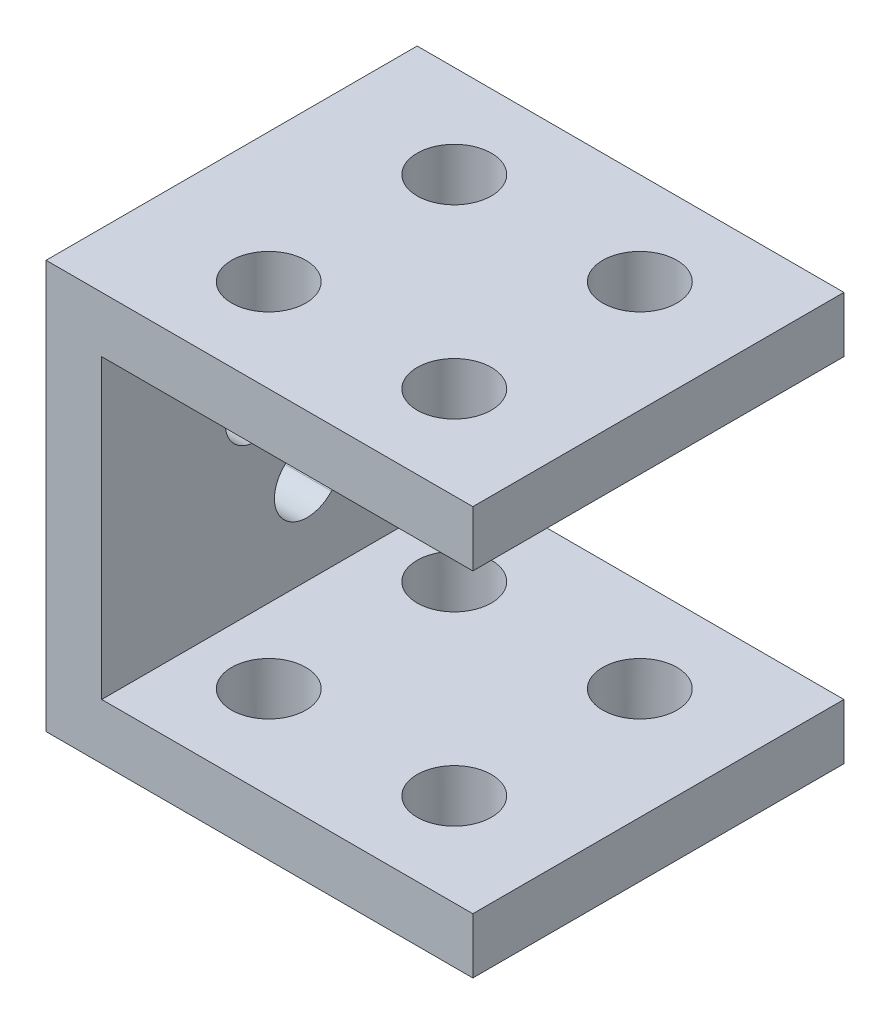
from build123d import *

# Parameters (mm, degrees)
BOSS_EXTRUDE1_DEPTH = 100
SKETCH2_R           = 10
CUT_EXTRUDE1_DEPTH  = 500
CUT_EXTRUDE2_DEPTH  = 500


with BuildPart() as part:
    # Sketch1 → Boss-Extrude1 (new body)
    with BuildSketch(Plane.XY):
        Polygon((0, 0), (100, 0), (100, -15), (-15, -15), (-15, 95), (100, 95), (100, 80), (0, 80), align=None)
    extrude(amount=BOSS_EXTRUDE1_DEPTH)

    # Sketch2 → Cut-Extrude1 (cut)
    with BuildSketch(Plane(origin=(0, 95, 0), x_dir=(1, 0, 0), z_dir=(0, 1, 0))):
        with Locations(Location((20, -25, 0), (0, 0, 270))):
            Circle(SKETCH2_R)
        with Locations(Location((70, -25, 0), (0, 0, 270))):
            Circle(SKETCH2_R)
        with Locations(Location((20, -75, 0), (0, 0, 270))):
            Circle(SKETCH2_R)
        with Locations(Location((70, -75, 0), (0, 0, 270))):
            Circle(SKETCH2_R)
    extrude(amount=-CUT_EXTRUDE1_DEPTH, mode=Mode.SUBTRACT)

    # Sketch3 → Cut-Extrude2 (cut)
    with BuildSketch(Plane(origin=(0, 0, 0), x_dir=(0, 0, -1), z_dir=(1, 0, 0))):
        with BuildLine():
            Line((-63.733404472, 53.788355895), (-44.717667379, 69.375025643))
            ThreePointArc((-44.717667379, 69.375025643), (-33.359667898, 68.249458127), (-34.485235414, 56.891458646))
            Line((-34.485235414, 56.891458646), (-53.500972507, 41.304788898))
            ThreePointArc((-53.500972507, 41.304788898), (-64.858971988, 42.430356414), (-63.733404472, 53.788355895))
        make_face()
        with BuildLine():
            Line((-51.188949328, 29.512455593), (-29.848080815, 53.133200052))
            ThreePointArc((-29.848080815, 53.133200052), (-17.387846498, 53.765023215), (-16.756023336, 41.304788898))
            Line((-16.756023336, 41.304788898), (-38.096891848, 17.684044439))
            ThreePointArc((-38.096891848, 17.684044439), (-50.557126165, 17.052221277), (-51.188949328, 29.512455593))
        make_face()
    extrude(amount=-CUT_EXTRUDE2_DEPTH, mode=Mode.SUBTRACT)


solid = part.part
